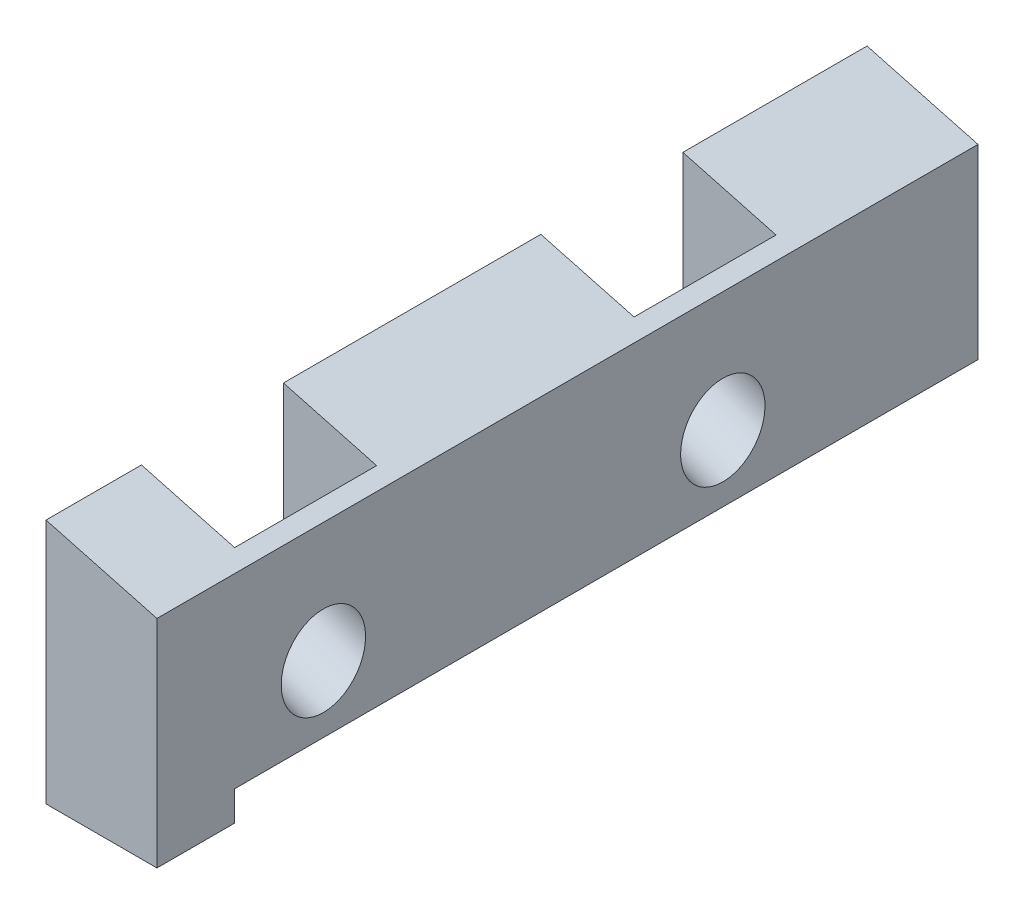
from build123d import *

# Parameters (mm, degrees)
BOSS_EXTRUDE1_DEPTH = 185
BOSS_EXTRUDE2_DEPTH = 35
CUT_EXTRUDE1_START  = 110
CUT_EXTRUDE1_DEPTH  = 32
CUT_EXTRUDE2_START  = -70
CUT_EXTRUDE2_DEPTH  = 32
SKETCH8_W           = 82.186037081
SKETCH8_H           = 19
LPATTERN1_COUNT     = 2
LPATTERN1_PITCH     = 180


with BuildPart() as part:
    # Sketch1 → Boss-Extrude1 (new, symmetric)
    with BuildSketch(Plane.XY):
        Polygon((0, 0), (50, 13.397459622), (50, 97.397459622), (0, 110.794919243), align=None)
    extrude(amount=BOSS_EXTRUDE1_DEPTH, both=True)

    # Sketch2 → Boss-Extrude2 (add)
    with BuildSketch(Plane.XY.offset(185)):
        Polygon((0, 0), (50, 0), (50, 13.397459622), align=None)
    extrude(amount=-BOSS_EXTRUDE2_DEPTH)

    # Sketch3 → Cut-Extrude1 (cut, symmetric)
    with BuildSketch(Plane.XY.offset(CUT_EXTRUDE1_START)):
        Polygon((16.51733163, 4.425805671), (42.003158605, 99.540206815), (0, 110.794919243), (0, 0), align=None)
    extrude(amount=CUT_EXTRUDE1_DEPTH, both=True, mode=Mode.SUBTRACT)

    # Sketch4 → Cut-Extrude2 (cut, symmetric)
    with BuildSketch(Plane.XY.offset(CUT_EXTRUDE2_START)):
        Polygon((16.51733163, 4.425805671), (0, 0), (0, 110.794919243), (42.003158605, 99.540206815), align=None)
    extrude(amount=CUT_EXTRUDE2_DEPTH, both=True, mode=Mode.SUBTRACT)

    # Sketch8 → Cut-Revolve1 (revolve, cut)
    with BuildSketch(Plane(origin=(19.79656359, 54.390611447, 0), x_dir=(-0.9396926207859083, 0.3420201433256693, 0), z_dir=(0.3420201433256693, 0.9396926207859083, 0)), mode=Mode.PRIVATE) as cut_revolve1_sk:
        with Locations((-10.891297764, -60.5)):
            Rectangle(SKETCH8_W, SKETCH8_H)
    cut_revolve1 = revolve(cut_revolve1_sk.sketch.rotate(Axis((24.894680211, 52.535048747, -70), (-0.9396926207859082, 0.3420201433256693, 0)), 270), axis=Axis((24.894680211, 52.535048747, -70), (-0.9396926207859082, 0.3420201433256693, 0)), mode=Mode.SUBTRACT)

    # LPattern1: Cut-Revolve1 ×2
    with Locations(*[(0, 0, i * LPATTERN1_PITCH) for i in range(1, LPATTERN1_COUNT)]):
        add(cut_revolve1, mode=Mode.SUBTRACT)


solid = part.part
